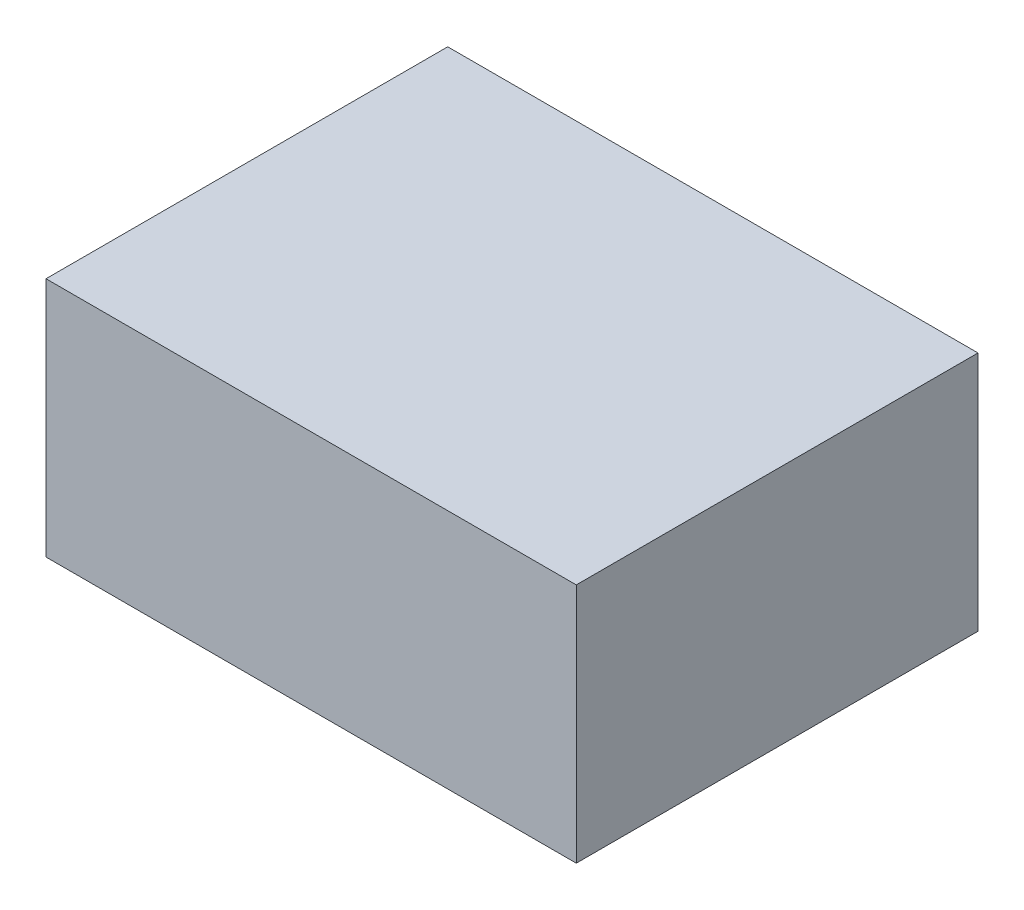
from build123d import *

# Parameters (mm, degrees)
SKETCH_1_W      = 660
SKETCH_1_H      = 300
EXTRUDE_1_DEPTH = 500
SHELL_1_T       = -10


with BuildPart() as part:
    # 草图1 → 凸台-拉伸1 (new body)
    with BuildSketch(Plane.XY):
        with Locations((-674.904398529, 2868.914811934)):
            Rectangle(SKETCH_1_W, SKETCH_1_H)
    extrude(amount=EXTRUDE_1_DEPTH)

    # 抽壳1
    shell_1_openings = [part.faces().sort_by_distance(p)[0] for p in [
        (-674.904398529, 2868.914811934, 0),
    ]]
    offset(amount=SHELL_1_T, openings=shell_1_openings, kind=Kind.INTERSECTION)


solid = part.part
